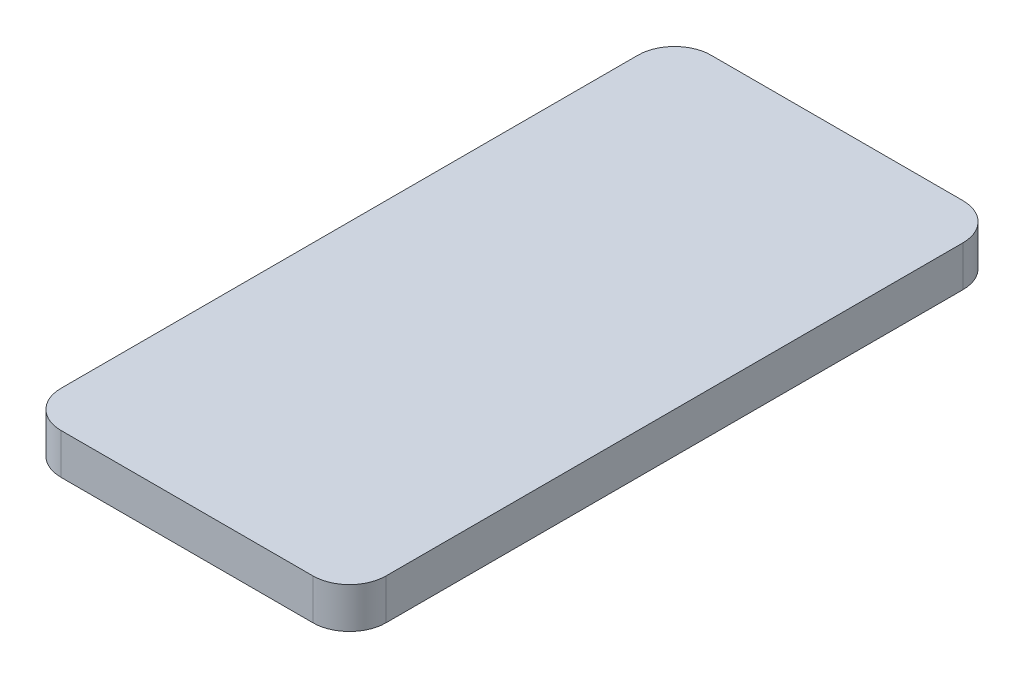
SolidWorks part; units mm, degrees
material "黑色POM "
ref_plane "前基準面" through (0, 0, 0) normal (0, 0, 1) x (1, 0, 0)
ref_plane "上基準面" through (0, 0, 0) normal (0, 1, 0) x (1, 0, 0)
ref_plane "右基準面" through (0, 0, 0) normal (1, 0, 0) x (0, 0, -1)
sketch "草图1" plane through (0, 0, 0) normal (0, 1, 0) x (1, 0, 0)
  line L1 (-20, -40) -> (20, -40)
  line L2 (-20, -40) -> (-20, 40)
  line L3 (-20, 40) -> (20, 40)
  line L4 (20, -40) -> (20, 40)
  line L5 (-20, -40) -> (20, 40) construction
  line L6 (-20, 40) -> (20, -40) construction
  point P0 (0, 0)
  dimension "D1" = 40
  dimension "D2" = 80
extrude "凸台-拉伸1" add sketch "草图1" along normal mid plane 5
fillet "圆角1" radius 4.5 4 edges at (20, 0, -40) (20, 0, 40) (-20, 0, -40) (-20, 0, 40)
